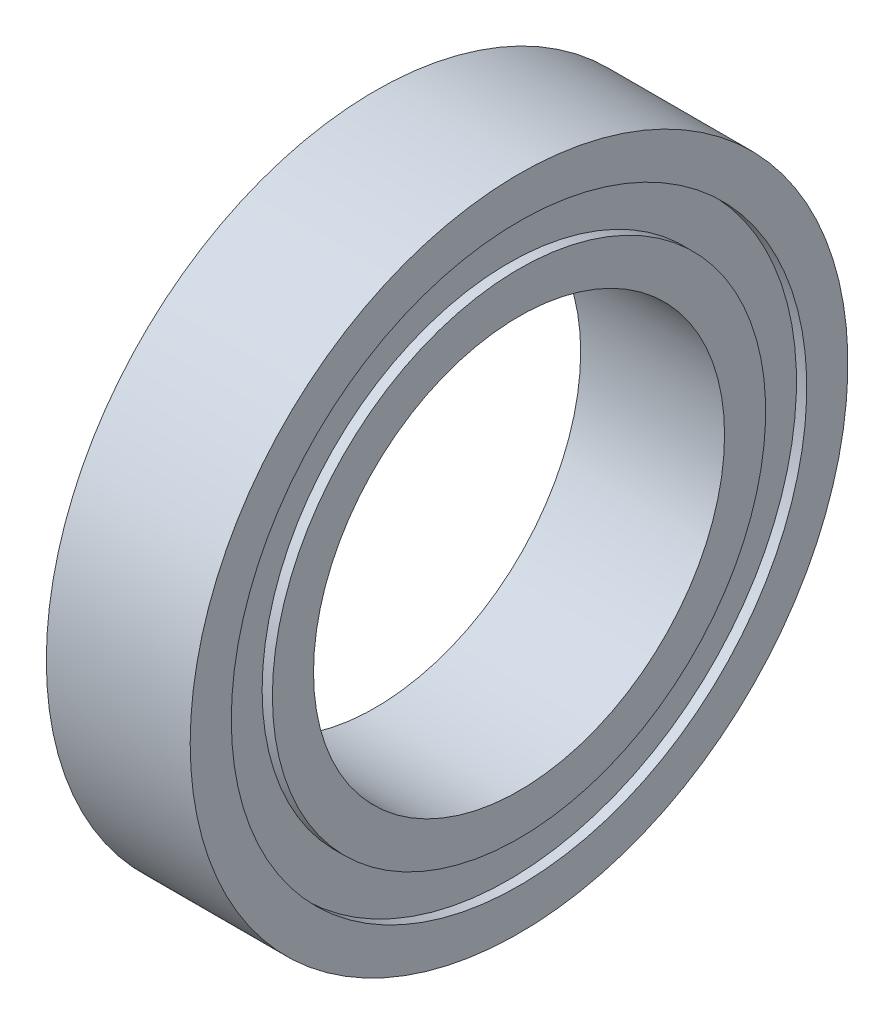
SolidWorks part; units mm, degrees
ref_plane "Front Plane" through (0, 0, 0) normal (0, 0, 1) x (1, 0, 0)
ref_plane "Top Plane" through (0, 0, 0) normal (0, 1, 0) x (1, 0, 0)
ref_plane "Right Plane" through (0, 0, 0) normal (1, 0, 0) x (0, 0, -1)
sketch "Sketch1" plane through (0, 0, 0) normal (0, 0, 1) x (1, 0, 0)
  line L0 (0, 0) -> (53.2336, 0) construction
  line L1 (14.6444, 14) -> (14.6444, 16)
  line L2 (14.6444, 10) -> (21.6444, 10)
  line L3 (14.6444, 10) -> (14.6444, 12)
  line L4 (14.6444, 16) -> (21.6444, 16)
  line L5 (21.6444, 10) -> (21.6444, 12)
  line L6 (14.6444, 12) -> (15.1444, 12)
  line L7 (21.6444, 14) -> (21.6444, 16)
  line L8 (14.6444, 14) -> (15.1444, 14)
  line L9 (15.1444, 12) -> (15.1444, 14)
  line L10 (21.6444, 12) -> (21.1444, 12)
  line L12 (21.6444, 14) -> (21.1444, 14)
  line L13 (21.1444, 12) -> (21.1444, 14)
  dimension "D1" = 7
  dimension "D2" = 20
  dimension "D3" = 32
  dimension "D4" = 0.5
  dimension "D5" = 2
revolve "Revolve1" add sketch "Sketch1" angle 360 about L0
